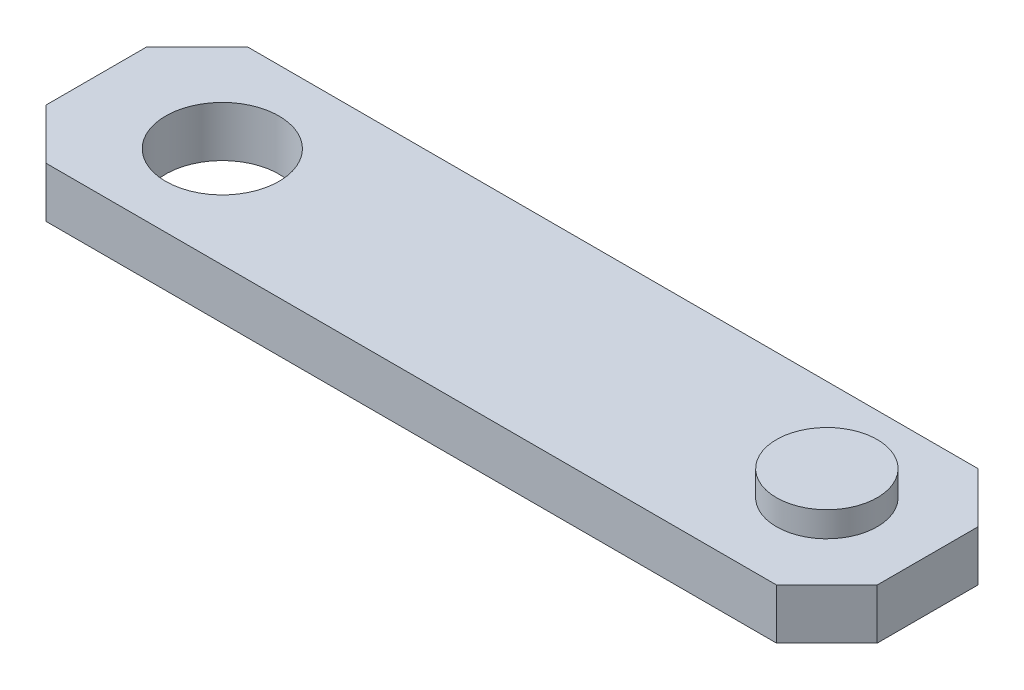
from build123d import *

# Parameters (mm, degrees)
SKETCH1_W           = 33
SKETCH1_H           = 8
BOSS_EXTRUDE1_DEPTH = 2
SKETCH2_R           = 2.25
CUT_EXTRUDE1_DEPTH  = 25.560457127
SKETCH3_R           = 2
BOSS_EXTRUDE2_DEPTH = 1
CHAMFER2_SIZE       = 2


with BuildPart() as part:
    # Sketch1 → Boss-Extrude1 (new body)
    with BuildSketch(Plane(origin=(0, 0, 0), x_dir=(1, 0, 0), z_dir=(0, 1, 0))):
        with Locations((6.806648575, 3.484396201)):
            Rectangle(SKETCH1_W, SKETCH1_H)
    extrude(amount=BOSS_EXTRUDE1_DEPTH)

    # Sketch2 → Cut-Extrude1 (cut, through all)
    with BuildSketch(Plane(origin=(0, 2, 0), x_dir=(1, 0, 0), z_dir=(0, 1, 0))):
        with Locations(Location((-4.693351425, 3.484396201, 0), (0, 0, 270))):
            Circle(SKETCH2_R)
    extrude(amount=-CUT_EXTRUDE1_DEPTH, mode=Mode.SUBTRACT)

    # Sketch3 → Boss-Extrude2 (add)
    with BuildSketch(Plane(origin=(0, 2, 0), x_dir=(1, 0, 0), z_dir=(0, 1, 0))):
        with Locations(Location((19.306648575, 3.484396201, 0), (0, 0, 270))):
            Circle(SKETCH3_R)
    extrude(amount=BOSS_EXTRUDE2_DEPTH)

    # Chamfer2
    chamfer2_edges = [part.edges().sort_by_distance(p)[0] for p in [
        (-9.693351425, 1, -7.484396201),
        (23.306648575, 1, -7.484396201),
        (23.306648575, 1, 0.515603799),
        (-9.693351425, 1, 0.515603799),
    ]]
    chamfer(chamfer2_edges, length=CHAMFER2_SIZE)


solid = part.part
